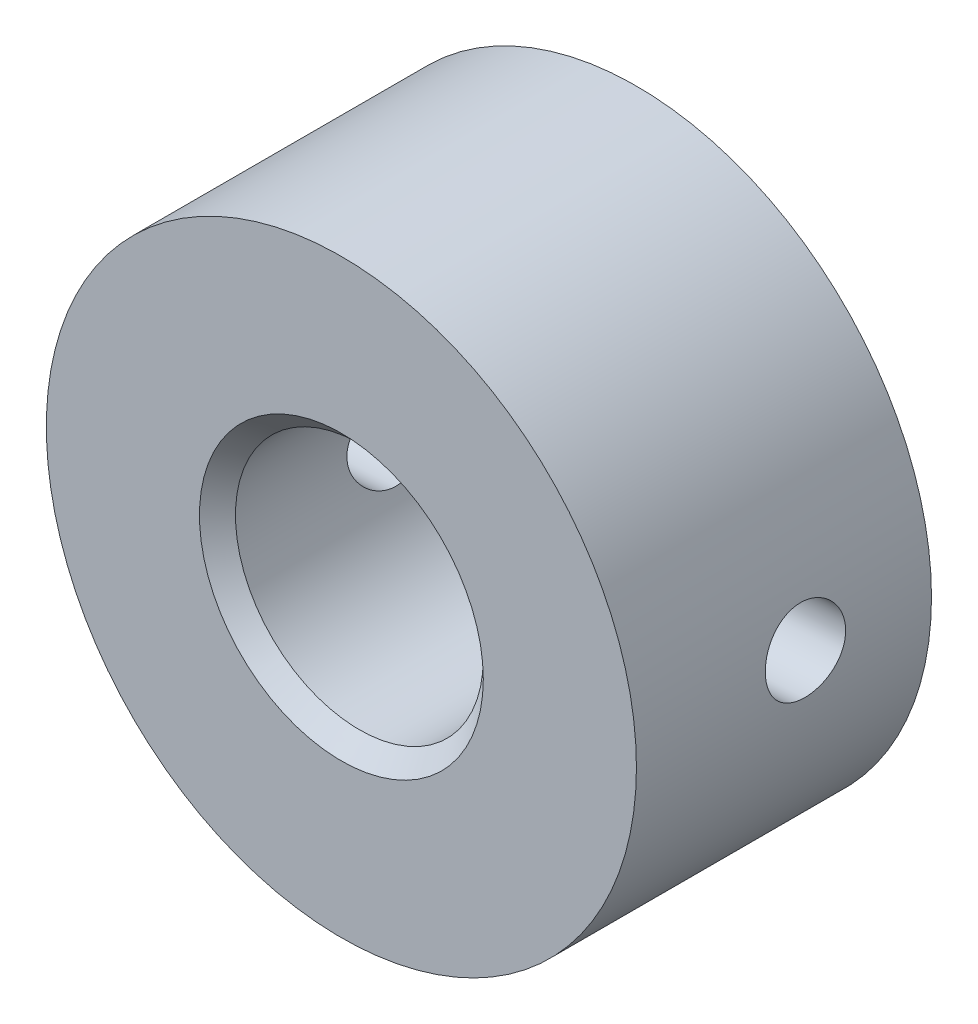
from build123d import *

# Parameters (mm, degrees)
SKETCH1_R                    = 25
BOSS_EXTRUDE1_DEPTH          = 25
M24_TAPPED_HOLE1_D           = 21
M24_TAPPED_HOLE1_DEPTH       = 57
M24_TAPPED_HOLE1_CSINK_D     = 24.05
M24_TAPPED_HOLE1_CSINK_ANGLE = 90
M24_TAPPED_HOLE1_TIP         = 6.3090365
M8_TAPPED_HOLE1_D            = 6.8
M8_TAPPED_HOLE1_DEPTH        = 63.75
M8_TAPPED_HOLE1_CSINK_D      = 8.05
M8_TAPPED_HOLE1_CSINK_ANGLE  = 90
M8_TAPPED_HOLE1_TIP          = 2.042926105


with BuildPart() as part:
    # Sketch1 → Boss-Extrude1 (new body)
    with BuildSketch(Plane.XY):
        Circle(SKETCH1_R)
    extrude(amount=BOSS_EXTRUDE1_DEPTH)

    # M24 Tapped Hole1
    with Locations(Plane.XY.offset(25)):
        with Locations((0, 0)):
            CounterSinkHole(M24_TAPPED_HOLE1_D / 2, M24_TAPPED_HOLE1_CSINK_D / 2, depth=M24_TAPPED_HOLE1_DEPTH, counter_sink_angle=M24_TAPPED_HOLE1_CSINK_ANGLE)
            with Locations((0, 0, -(M24_TAPPED_HOLE1_DEPTH + M24_TAPPED_HOLE1_TIP / 2))):  # 118° drill point
                Cone(0, M24_TAPPED_HOLE1_D / 2, M24_TAPPED_HOLE1_TIP, mode=Mode.SUBTRACT)

    # M8 Tapped Hole1
    with Locations(Plane(origin=(-24.965469306, -1.313522862, 10.643433194), x_dir=(0.052540914496, -0.998618772257, 0), z_dir=(-0.998618772257, -0.052540914496, 0))):
        with Locations((0, 0)):
            CounterSinkHole(M8_TAPPED_HOLE1_D / 2, M8_TAPPED_HOLE1_CSINK_D / 2, depth=M8_TAPPED_HOLE1_DEPTH, counter_sink_angle=M8_TAPPED_HOLE1_CSINK_ANGLE)
            with Locations((0, 0, -(M8_TAPPED_HOLE1_DEPTH + M8_TAPPED_HOLE1_TIP / 2))):  # 118° drill point
                Cone(0, M8_TAPPED_HOLE1_D / 2, M8_TAPPED_HOLE1_TIP, mode=Mode.SUBTRACT)


solid = part.part
